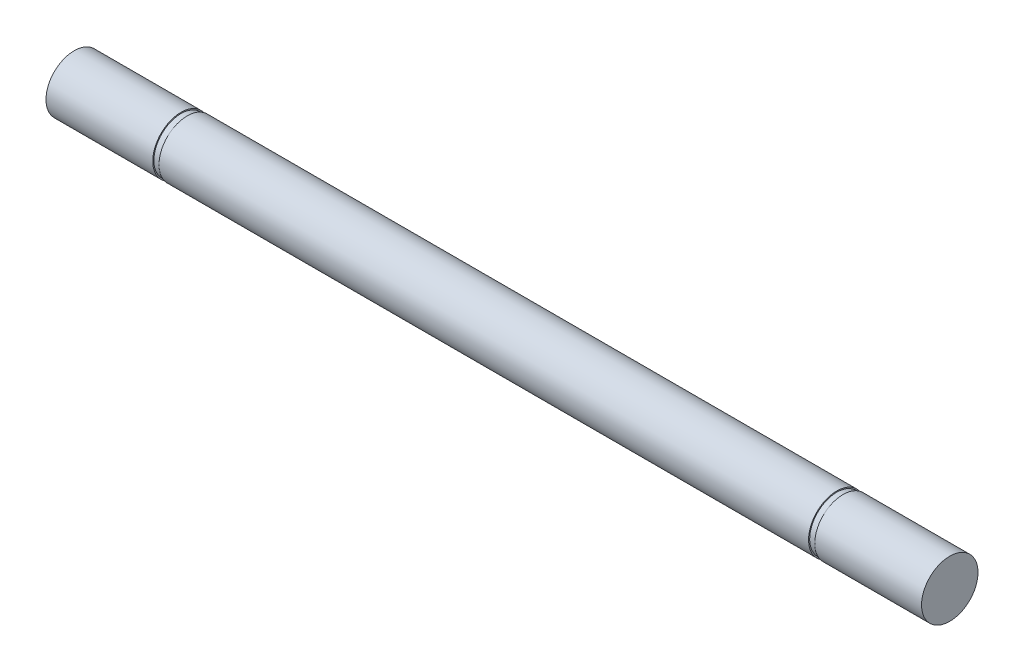
SolidWorks part; units mm, degrees
ref_plane "Front Plane" through (0, 0, 0) normal (0, 0, 1) x (1, 0, 0)
ref_plane "Top Plane" through (0, 0, 0) normal (0, 1, 0) x (1, 0, 0)
ref_plane "Right Plane" through (0, 0, 0) normal (1, 0, 0) x (0, 0, -1)
sketch "Sketch1" plane through (0, 0, 0) normal (0, 0, 1) x (1, 0, 0)
  line L0 (-57.5963, -12.1065) -> (-57.5963, -7.1065)
  line L1 (-57.5963, -7.1065) -> (-38.6963, -7.1065)
  line L2 (97.4037, -7.1065) -> (97.4037, -12.1065)
  line L3 (97.4037, -12.1065) -> (-57.5963, -12.1065)
  line L4 (78.5037, -7.1065) -> (97.4037, -7.1065)
  line L6 (-38.6963, -7.1065) -> (-38.6963, -7.3065)
  line L7 (-38.6963, -7.3065) -> (-37.5963, -7.3065)
  line L8 (-37.5963, -7.1065) -> (-37.5963, -7.3065)
  line L9 (-37.5963, -7.1065) -> (77.4037, -7.1065)
  line L10 (77.4037, -7.1065) -> (77.4037, -7.3065)
  line L11 (77.4037, -7.3065) -> (78.5037, -7.3065)
  line L12 (78.5037, -7.1065) -> (78.5037, -7.3065)
  dimension "D1" = 5
  dimension "D2" = 0.2
  dimension "D3" = 1.1
  dimension "D4" = 0.2
  dimension "D5" = 1.1
  dimension "D6" = 115
  dimension "D7" = 155
  dimension "D8" = 20
revolve "Revolve1" add sketch "Sketch1" angle 360 about L3
